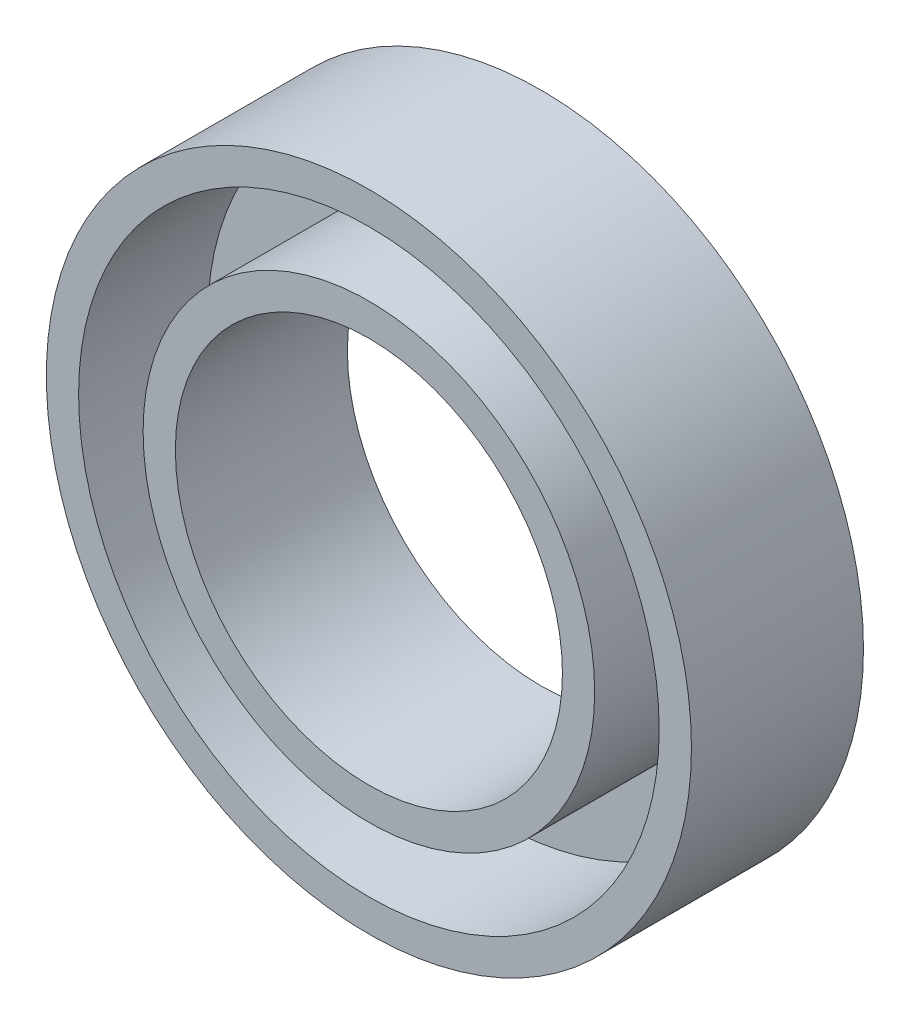
from build123d import *

# Parameters (mm, degrees)
SKETCH1_R           = 15
SKETCH1_R_2         = 9
BOSS_EXTRUDE1_DEPTH = 8
SKETCH2_R           = 13.5
SKETCH2_R_2         = 10.5
CUT_EXTRUDE1_DEPTH  = 6


with BuildPart() as part:
    # Sketch1 → Boss-Extrude1 (new body)
    with BuildSketch(Plane.XY):
        Circle(SKETCH1_R)
        Circle(SKETCH1_R_2, mode=Mode.SUBTRACT)
    extrude(amount=BOSS_EXTRUDE1_DEPTH)

    # Sketch2 → Cut-Extrude1 (cut)
    with BuildSketch(Plane.XY.offset(8)):
        Circle(SKETCH2_R)
        Circle(SKETCH2_R_2, mode=Mode.SUBTRACT)
    extrude(amount=-CUT_EXTRUDE1_DEPTH, mode=Mode.SUBTRACT)


solid = part.part
